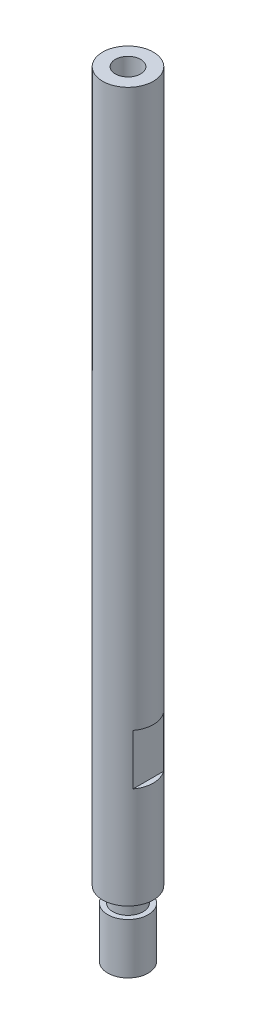
from build123d import *

# Parameters (mm, degrees)
CUT_EXTRUDE1_DEPTH      = 140.008995048
CUT_EXTRUDE1_DEPTH_BACK = 140.008995048
SKETCH2_W               = 1
SKETCH2_H               = 10
M6_TAPPED_HOLE1_D       = 5
M6_TAPPED_HOLE1_DEPTH   = 12
M6_TAPPED_HOLE1_TIP     = 1.502151548


with BuildPart() as part:
    # Sketch1 → Revolve1 (revolve)
    with BuildSketch(Plane.XY):
        Polygon((0, 14.170965918), (0, -138.829034082), (-4, -138.829034082), (-4, -128.829034082), (-3, -128.829034082), (-3, -125.829034082), (-5, -125.829034082), (-5, 14.170965918), align=None)
    revolve(axis=Axis((0, 14.170965918, 0), (0, -1, 0)))

    # Sketch2 → Cut-Extrude1 (cut, two sides: drawn at the far end of the back side and taken through both)
    with BuildSketch(Plane.XY.offset(-CUT_EXTRUDE1_DEPTH_BACK)):
        with Locations((-4.5, -100.829034082)):
            Rectangle(SKETCH2_W, SKETCH2_H)
        with Locations((4.5, -100.829034082)):
            Rectangle(SKETCH2_W, SKETCH2_H)
    extrude(amount=CUT_EXTRUDE1_DEPTH + CUT_EXTRUDE1_DEPTH_BACK, mode=Mode.SUBTRACT)

    # M6 Tapped Hole1
    with Locations(Plane(origin=(0, 14.170965918, 0), x_dir=(1, 0, 0), z_dir=(0, 1, 0))):
        with Locations((0, 0)):
            Hole(M6_TAPPED_HOLE1_D / 2, depth=M6_TAPPED_HOLE1_DEPTH)
            with Locations((0, 0, -(M6_TAPPED_HOLE1_DEPTH + M6_TAPPED_HOLE1_TIP / 2))):  # 118° drill point
                Cone(0, M6_TAPPED_HOLE1_D / 2, M6_TAPPED_HOLE1_TIP, mode=Mode.SUBTRACT)


solid = part.part
